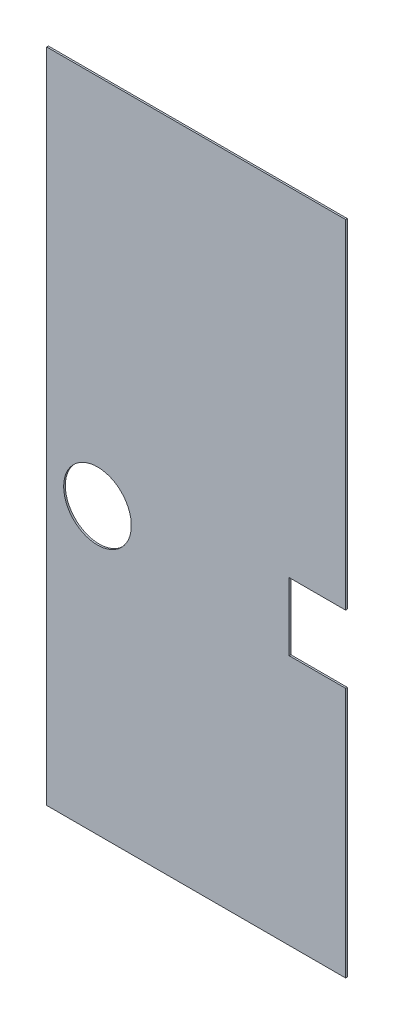
from build123d import *

# Parameters (mm, degrees)
SKETCH1_W           = 530
SKETCH1_H           = 1165
BOSS_EXTRUDE1_DEPTH = 3
SKETCH2_R           = 60
SKETCH2_W           = 120
SKETCH2_H           = 120
CUT_EXTRUDE1_DEPTH  = 10


with BuildPart() as part:
    # Sketch1 → Boss-Extrude1 (new body)
    with BuildSketch(Plane.XY):
        with Locations((265, 582.5)):
            Rectangle(SKETCH1_W, SKETCH1_H)
    extrude(amount=BOSS_EXTRUDE1_DEPTH)

    # Sketch2 → Cut-Extrude1 (cut)
    with BuildSketch(Plane(origin=(0, 0, 0), x_dir=(-1, 0, 0), z_dir=(0, 0, -1))):
        with Locations((-90, 505)):
            Circle(SKETCH2_R)
        with Locations((-490, 505)):
            Rectangle(SKETCH2_W, SKETCH2_H)
    extrude(amount=-CUT_EXTRUDE1_DEPTH, mode=Mode.SUBTRACT)


solid = part.part
